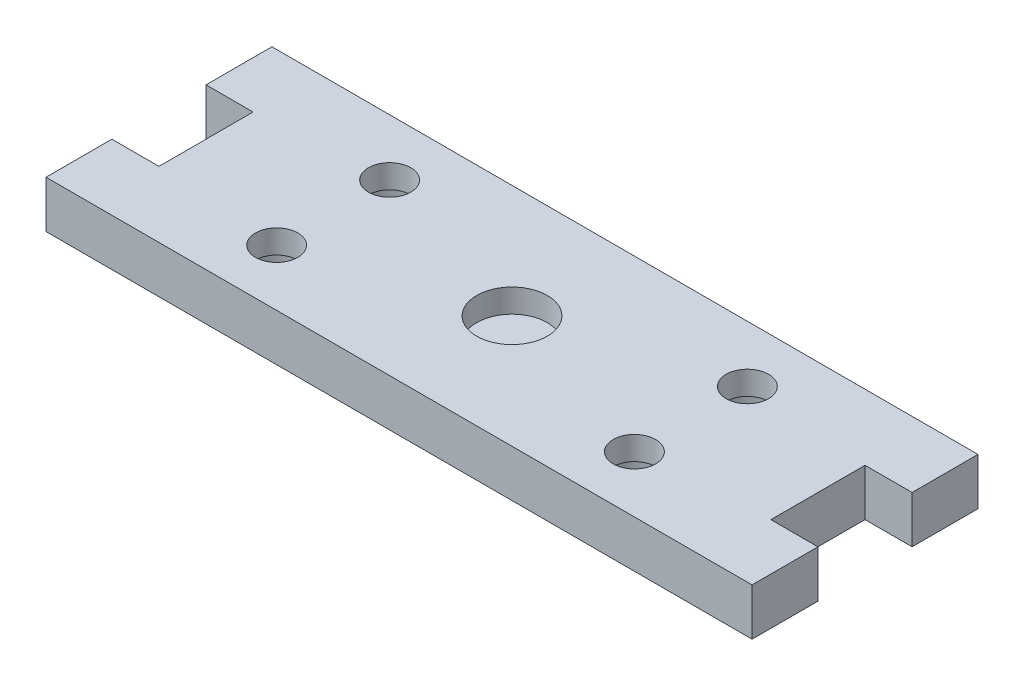
from build123d import *

# Parameters (mm, degrees)
SKETCH1_W                                  = 150
SKETCH1_H                                  = 48
BOSS_EXTRUDE1_DEPTH                        = 10
CBORE_FOR_M8_CHEESE_HEAD_SCREW1_AT_2_COUNT = 2
CBORE_FOR_M8_CHEESE_HEAD_SCREW1_AT_2_PITCH = 76
CBORE_FOR_M8_CHEESE_HEAD_SCREW1_AT_3_COUNT = 2
CBORE_FOR_M8_CHEESE_HEAD_SCREW1_AT_3_PITCH = 24
CBORE_FOR_M8_CHEESE_HEAD_SCREW1_AT_4_COUNT = 2
CBORE_FOR_M8_CHEESE_HEAD_SCREW1_AT_4_PITCH = 79.699435381
SKETCH6_R                                  = 7.5
CUT_EXTRUDE2_DEPTH                         = 5
SKETCH7_W                                  = 20
SKETCH7_H                                  = 20
CUT_EXTRUDE3_DEPTH                         = 80.37883849


with BuildPart() as part:
    # Sketch1 → Boss-Extrude1 (new body)
    with BuildSketch(Plane(origin=(0, 0, 0), x_dir=(1, 0, 0), z_dir=(0, 1, 0))):
        Rectangle(SKETCH1_W, SKETCH1_H)
    extrude(amount=BOSS_EXTRUDE1_DEPTH)

    # Sketch4 → CBORE for M8 Cheese Head Screw1 (revolve, cut)
    with BuildSketch(Plane(origin=(38, 0, 12), x_dir=(0, 0, -1), z_dir=(1, 0, 0))):
        Polygon((0, 0), (0, 12.703872786), (4.5, 10), (4.5, 5), (7.5, 5), (7.5, 0.025), (7.525, 0), align=None)
    cbore_for_m8_cheese_head_screw1 = revolve(axis=Axis((38, -6.35, 12), (0, 1, 0)), mode=Mode.SUBTRACT)

    # CBORE for M8 Cheese Head Screw1 at 2: CBORE for M8 Cheese Head Screw1 ×2
    with Locations(*[(-i * CBORE_FOR_M8_CHEESE_HEAD_SCREW1_AT_2_PITCH, 0, 0) for i in range(1, CBORE_FOR_M8_CHEESE_HEAD_SCREW1_AT_2_COUNT)]):
        add(cbore_for_m8_cheese_head_screw1, mode=Mode.SUBTRACT)

    # CBORE for M8 Cheese Head Screw1 at 3: CBORE for M8 Cheese Head Screw1 ×2
    with Locations(*[(0, 0, -i * CBORE_FOR_M8_CHEESE_HEAD_SCREW1_AT_3_PITCH) for i in range(1, CBORE_FOR_M8_CHEESE_HEAD_SCREW1_AT_3_COUNT)]):
        add(cbore_for_m8_cheese_head_screw1, mode=Mode.SUBTRACT)

    # CBORE for M8 Cheese Head Screw1 at 4: CBORE for M8 Cheese Head Screw1 ×2
    with Locations(*[Vector(-0.9535826651341417, 0, -0.3011313679370974) * (i * CBORE_FOR_M8_CHEESE_HEAD_SCREW1_AT_4_PITCH) for i in range(1, CBORE_FOR_M8_CHEESE_HEAD_SCREW1_AT_4_COUNT)]):
        add(cbore_for_m8_cheese_head_screw1, mode=Mode.SUBTRACT)

    # Sketch6 → Cut-Extrude2 (cut)
    with BuildSketch(Plane(origin=(0, 10, 0), x_dir=(1, 0, 0), z_dir=(0, 1, 0))):
        with Locations(Location((0, 0, 0), (0, 0, 270))):
            Circle(SKETCH6_R)
    extrude(amount=-CUT_EXTRUDE2_DEPTH, mode=Mode.SUBTRACT)

    # Sketch7 → Cut-Extrude3 (cut, through all)
    with BuildSketch(Plane(origin=(0, 10, 0), x_dir=(1, 0, 0), z_dir=(0, 1, 0))):
        with Locations((75, 0)):
            Rectangle(SKETCH7_W, SKETCH7_H)
        with Locations((-75, 0)):
            Rectangle(SKETCH7_W, SKETCH7_H)
    extrude(amount=-CUT_EXTRUDE3_DEPTH, mode=Mode.SUBTRACT)


solid = part.part
